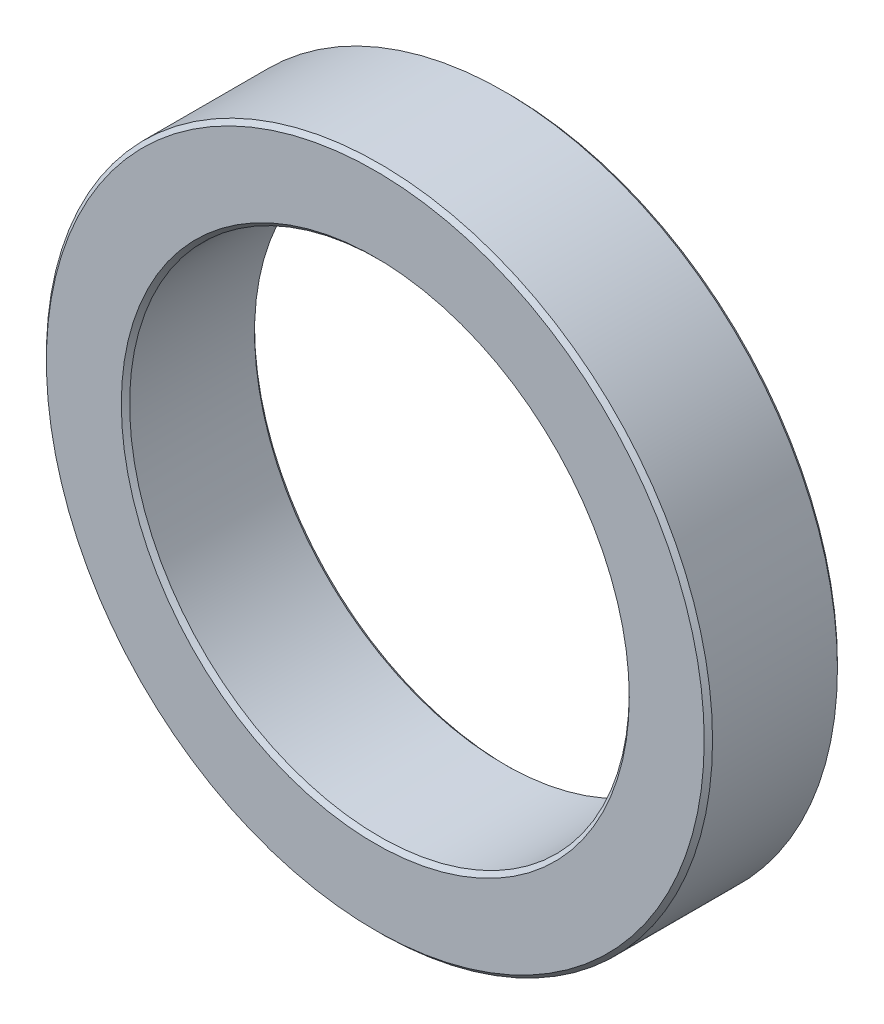
from build123d import *

# Parameters (mm, degrees)
SKETCH1_R           = 40
SKETCH1_R_2         = 30
BOSS_EXTRUDE1_DEPTH = 16
CHAMFER1_SIZE       = 0.5


with BuildPart() as part:
    # Sketch1 → Boss-Extrude1 (new body)
    with BuildSketch(Plane.XY):
        Circle(SKETCH1_R)
        Circle(SKETCH1_R_2, mode=Mode.SUBTRACT)
    extrude(amount=BOSS_EXTRUDE1_DEPTH)

    # Chamfer1
    chamfer1_edges = [part.edges().sort_by_distance(p)[0] for p in [
        (-40, 0, 0),
        (-40, 0, 16),
        (-30, 0, 0),
        (-30, 0, 16),
    ]]
    chamfer(chamfer1_edges, length=CHAMFER1_SIZE)


solid = part.part
